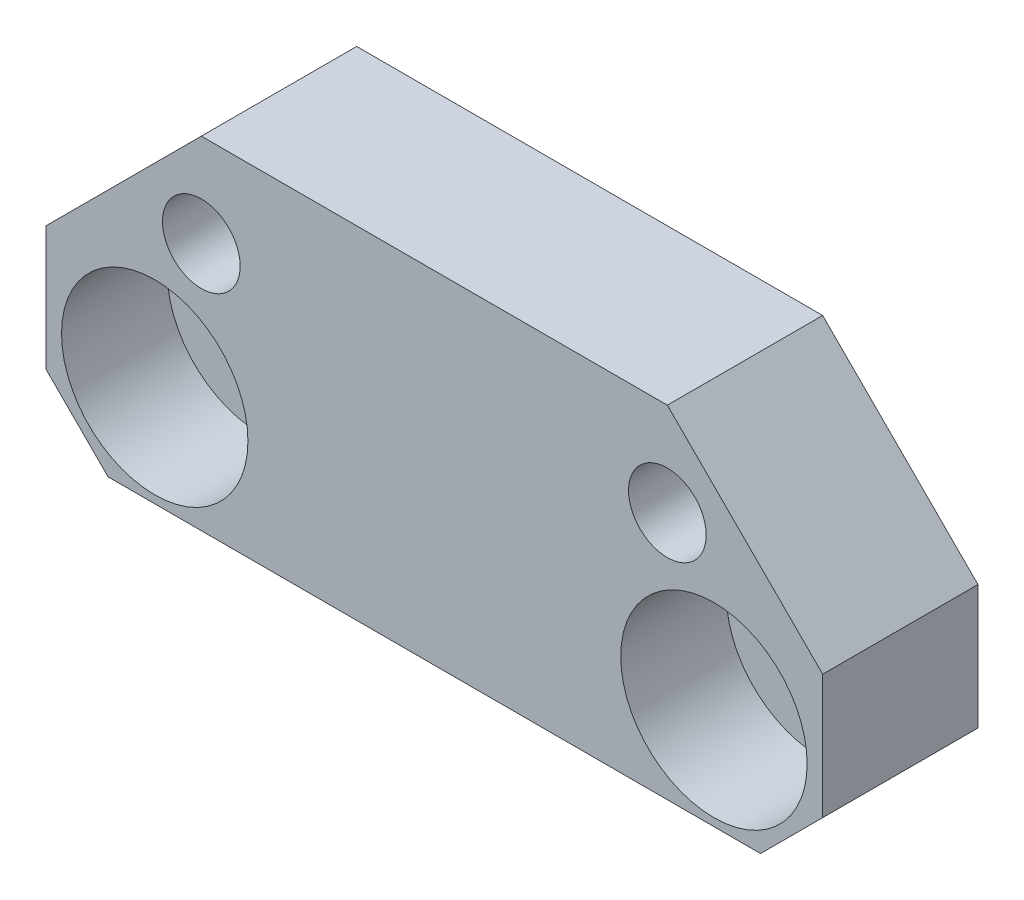
from build123d import *

# Parameters (mm, degrees)
SKETCH1_W                                           = 8.5
SKETCH1_H                                           = 3.5
BOSS_EXTRUDE1_DEPTH                                 = 2.5
M3_TAPPED_HOLE1_D                                   = 2.5
HOLE_SIZE_BY_SOCKET_HEAD_CAP_SCREW_TYPE_D           = 3.4
HOLE_SIZE_BY_SOCKET_HEAD_CAP_SCREW_TYPE_CBORE_D     = 6
HOLE_SIZE_BY_SOCKET_HEAD_CAP_SCREW_TYPE_CBORE_DEPTH = 3.4
CHAMFER2_SIZE                                       = 5
CHAMFER3_SIZE                                       = 2


with BuildPart() as part:
    # Sketch1 → Boss-Extrude1 (new, symmetric)
    with BuildSketch(Plane.XY):
        Polygon((-12.5, 2), (-12.5, -5.5), (12.5, -5.5), (12.5, 2), (4, 2), (4, 5.5), (-4, 5.5), (-4, 2), align=None)
        with Locations((8.25, 3.75)):
            Rectangle(SKETCH1_W, SKETCH1_H)
        with Locations((-8.25, 3.75)):
            Rectangle(SKETCH1_W, SKETCH1_H)
    extrude(amount=BOSS_EXTRUDE1_DEPTH, both=True)

    # M3 Tapped Hole1 (through all)
    with Locations(Plane.XY.offset(2.5)):
        with Locations((-7.5, 2.5), (7.5, 2.5)):
            Hole(M3_TAPPED_HOLE1_D / 2)

    # Hole size (by socket head cap screw type)1 (through all)
    with Locations(Plane.XY.offset(2.5)):
        with Locations((9, -2.25), (-9, -2.25)):
            CounterBoreHole(HOLE_SIZE_BY_SOCKET_HEAD_CAP_SCREW_TYPE_D / 2, HOLE_SIZE_BY_SOCKET_HEAD_CAP_SCREW_TYPE_CBORE_D / 2, HOLE_SIZE_BY_SOCKET_HEAD_CAP_SCREW_TYPE_CBORE_DEPTH)

    # Chamfer2
    chamfer2_edges = [part.edges().sort_by_distance(p)[0] for p in [
        (12.5, 5.5, 0),
        (-12.5, 5.5, 0),
    ]]
    chamfer(chamfer2_edges, length=CHAMFER2_SIZE)

    # Chamfer3
    chamfer3_edges = [part.edges().sort_by_distance(p)[0] for p in [
        (12.5, -5.5, 0),
        (-12.5, -5.5, 0),
    ]]
    chamfer(chamfer3_edges, length=CHAMFER3_SIZE)


solid = part.part
